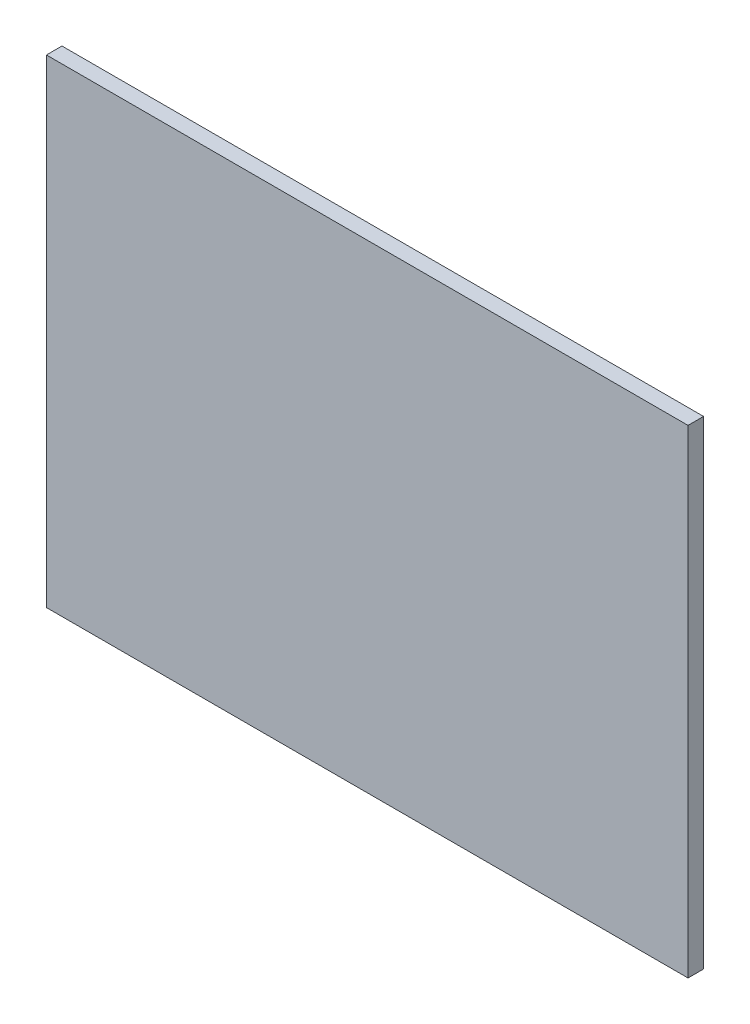
SolidWorks part; units mm, degrees
ref_plane "前视基准面" through (0, 0, 0) normal (0, 0, 1) x (1, 0, 0)
ref_plane "上视基准面" through (0, 0, 0) normal (0, 1, 0) x (1, 0, 0)
ref_plane "右视基准面" through (0, 0, 0) normal (1, 0, 0) x (0, 0, -1)
sketch "草图1" plane through (0, 0, 0) normal (0, 0, 1) x (1, 0, 0)
  line L1 (-124, -92.5) -> (124, -92.5)
  line L2 (-124, -92.5) -> (-124, 92.5)
  line L3 (-124, 92.5) -> (124, 92.5)
  line L4 (124, -92.5) -> (124, 92.5)
  line L5 (-124, -92.5) -> (124, 92.5) construction
  line L6 (-124, 92.5) -> (124, -92.5) construction
  point P0 (0, 0)
  dimension "D1" = 185
  dimension "D2" = 248
extrude "凸台-拉伸1" add sketch "草图1" along normal blind 6
